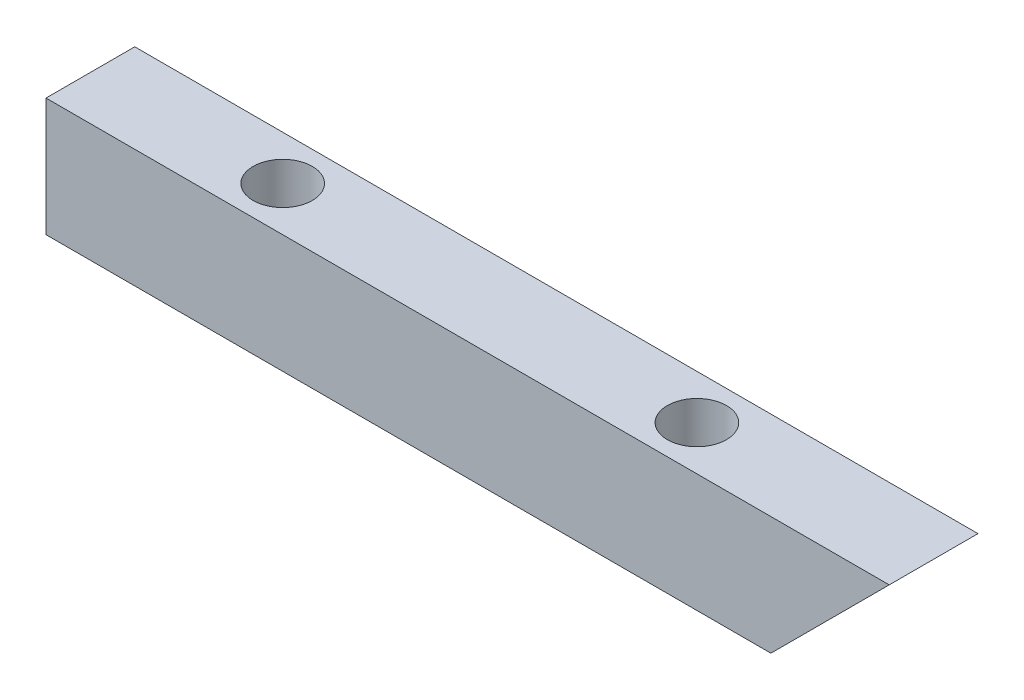
SolidWorks part; units mm, degrees
ref_plane "前视基准面" through (0, 0, 0) normal (0, 0, 1) x (1, 0, 0)
ref_plane "上视基准面" through (0, 0, 0) normal (0, 1, 0) x (1, 0, 0)
ref_plane "右视基准面" through (0, 0, 0) normal (1, 0, 0) x (0, 0, -1)
sketch "草图1" plane through (0, 0, 0) normal (0, 1, 0) x (1, 0, 0)
  line L1 (-135, -15) -> (135, -15)
  line L2 (-135, -15) -> (-135, 15)
  line L3 (-135, 15) -> (135, 15)
  line L4 (135, -15) -> (135, 15)
  line L5 (-135, -15) -> (135, 15) construction
  line L6 (-135, 15) -> (135, -15) construction
  point P0 (0, 0)
  dimension "D1" = 270
  dimension "D2" = 30
extrude "凸台-拉伸1" add sketch "草图1" along normal blind 40
sketch "草图2" plane through (0, 40, 0) normal (0, 1, 0) x (1, 0, 0)
  line L1 (0, 0) -> (0, 40) construction
  circle A0 centre (70, 0) radius 10
  circle A1 centre (-70, 0) radius 10
  dimension "D1" = 20
  dimension "D2" = 140
  dimension "D3" = 40
extrude "切除-拉伸2" cut sketch "草图2" against normal blind 30
sketch "草图3" plane through (135, 0, 0) normal (1, 0, 0) x (0, 0, -1)
  line L4 (-15, 0) -> (15, 0)
  line L5 (15, 0) -> (15, 40)
  line L6 (15, 40) -> (-15, 40)
  line L7 (-15, 40) -> (-15, 0)
  line L8 (-15, 0) -> (15, 0)
  line L9 (15, 0) -> (15, 40)
  line L10 (15, 40) -> (-15, 40)
  line L11 (-15, 40) -> (-15, 0)
  dimension "D1" = 0
extrude "凸台-拉伸2" add sketch "草图3" along normal blind 15
sketch "草图4" plane through (0, 0, 15) normal (0, 0, 1) x (1, 0, 0)
  line L0 (150, 40) -> (110, 0)
  line L1 (-135, 0) -> (150, 0) construction
  line L2 (150, 40) -> (150, 0) construction
  line L3 (150, 40) -> (150, 0)
  line L4 (110, 0) -> (150, 0)
  dimension "D1" = 45
extrude "切除-拉伸3" cut sketch "草图4" against normal through all
